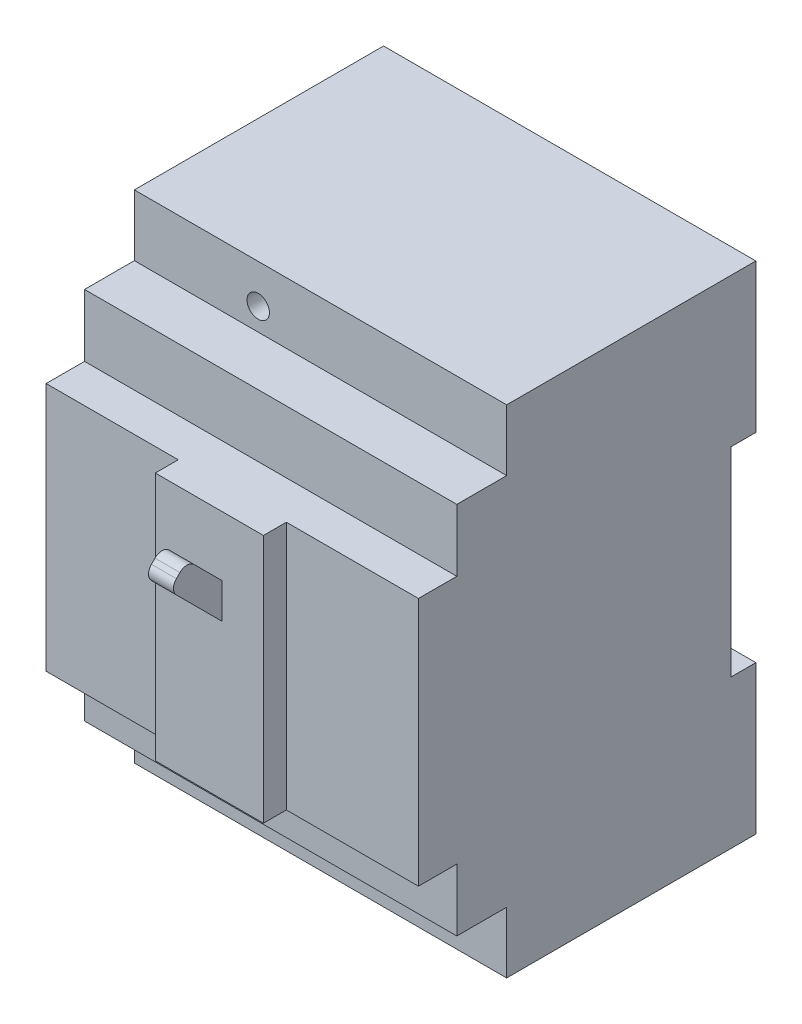
from build123d import *

# Parameters (mm, degrees)
SKETCH1_W                  = 74.7
SKETCH1_H                  = 99.6
BOSS_EXTRUDE1_DEPTH        = 33.85
F_4_5_4_5_DIAMETER_HOLE1_D = 4.5
SKETCH4_W                  = 74.7
SKETCH4_H                  = 12.3
CUT_EXTRUDE1_DEPTH         = 17.7
SKETCH5_W                  = 74.7
SKETCH5_H                  = 12.5
CUT_EXTRUDE2_DEPTH         = 7.7
SKETCH6_W                  = 21.7
SKETCH6_H                  = 50
BOSS_EXTRUDE2_DEPTH        = 4.6
SKETCH7_W                  = 5
SKETCH7_H                  = 40
CUT_EXTRUDE3_DEPTH         = 118.6
BOSS_EXTRUDE3_DEPTH        = 2.5
FILLET1_R                  = 2


with BuildPart() as part:
    # Sketch1 → Boss-Extrude1 (new, symmetric)
    with BuildSketch(Plane.XY):
        Rectangle(SKETCH1_W, SKETCH1_H)
    extrude(amount=BOSS_EXTRUDE1_DEPTH, both=True)

    # Ø4.5 (4.5) Diameter Hole1 (through all)
    with Locations(Plane.XY.offset(33.85)):
        with Locations((-12.5, 42), (12.5, -42)):
            Hole(F_4_5_4_5_DIAMETER_HOLE1_D / 2)

    # Sketch4 → Cut-Extrude1 (cut)
    with BuildSketch(Plane.XY.offset(33.85)):
        with Locations((0, 43.65)):
            Rectangle(SKETCH4_W, SKETCH4_H)
        with Locations((0, -43.65)):
            Rectangle(SKETCH4_W, SKETCH4_H)
    extrude(amount=-CUT_EXTRUDE1_DEPTH, mode=Mode.SUBTRACT)

    # Sketch5 → Cut-Extrude2 (cut)
    with BuildSketch(Plane.XY.offset(33.85)):
        with Locations((0, -31.25)):
            Rectangle(SKETCH5_W, SKETCH5_H)
        with Locations((0, 31.25)):
            Rectangle(SKETCH5_W, SKETCH5_H)
    extrude(amount=-CUT_EXTRUDE2_DEPTH, mode=Mode.SUBTRACT)

    # Sketch6 → Boss-Extrude2 (add)
    with BuildSketch(Plane.XY.offset(33.85)):
        Rectangle(SKETCH6_W, SKETCH6_H)
    extrude(amount=BOSS_EXTRUDE2_DEPTH)

    # Sketch7 → Cut-Extrude3 (cut)
    with BuildSketch(Plane(origin=(37.35, 0, 0), x_dir=(0, 0, -1), z_dir=(1, 0, 0))):
        with Locations((31.35, 0)):
            Rectangle(SKETCH7_W, SKETCH7_H)
    extrude(amount=-CUT_EXTRUDE3_DEPTH, mode=Mode.SUBTRACT)

    # Sketch8 → Boss-Extrude3 (add, symmetric)
    with BuildSketch(Plane(origin=(0, 0, 0), x_dir=(0, 0, -1), z_dir=(1, 0, 0))):
        Polygon((-38.45, 13), (-45.45, 20), (-48.985533906, 16.464466094), (-38.45, 5.928932188), align=None)
    extrude(amount=BOSS_EXTRUDE3_DEPTH, both=True)

    # Fillet1
    fillet1_edges = [part.edges().sort_by_distance(p)[0] for p in [
        (0, 20, 45.45),
        (0, 16.464466094, 48.985533906),
    ]]
    fillet(fillet1_edges, radius=FILLET1_R)


solid = part.part
